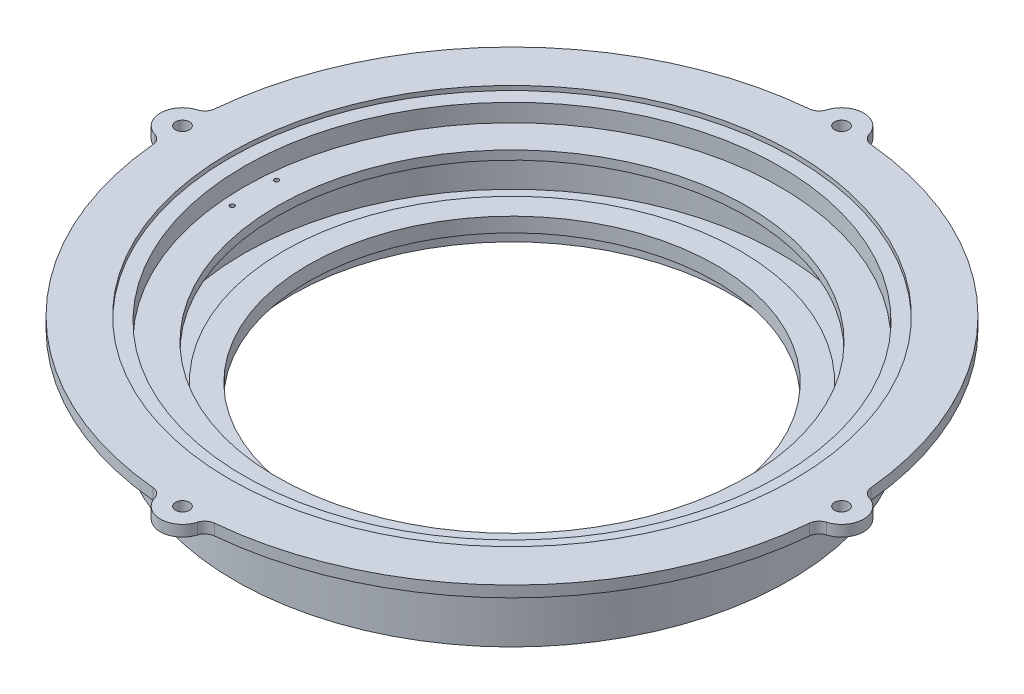
SolidWorks part; units mm, degrees
material "1060 合金"
ref_plane "Front Plane" through (0, 0, 0) normal (0, 0, 1) x (1, 0, 0)
ref_plane "Top Plane" through (0, 0, 0) normal (0, 1, 0) x (1, 0, 0)
ref_plane "Right Plane" through (0, 0, 0) normal (1, 0, 0) x (0, 0, -1)
sketch "Sketch1" plane through (0, 0, 0) normal (0, 0, 1) x (1, 0, 0)
  line L0 (0, 0) -> (0, -19.9402) construction
  line L1 (-125, 139.5) -> (-125, 175.5)
  line L2 (-125, 139.5) -> (-99, 139.5)
  line L3 (125, 139) -> (-125, 139) construction
  line L4 (-103, 144.5) -> (-103, 154.5)
  line L5 (-103, 154.5) -> (-92, 154.5)
  line L6 (-121, 180.5) -> (-148.7461, 180.5)
  line L7 (-148.7461, 180.5) -> (-148.7461, 175.5)
  line L8 (-148.7461, 175.5) -> (-125, 175.5)
  line L9 (-92, 154.5) -> (-92, 147.9626)
  line L10 (-92, 147.9626) -> (-99, 147.9626)
  line L11 (-99, 147.9626) -> (-99, 139.5)
  line L13 (-121, 170.5) -> (-106, 170.5)
  line L14 (-103, 144.5) -> (-121, 144.5)
  line L15 (-121, 144.5) -> (-121, 166.5)
  line L17 (-121, 166.5) -> (-106, 166.5)
  line L18 (-106, 170.5) -> (-106, 166.5)
  line L19 (-121, 170.5) -> (-121, 180.5)
  dimension "D1" = 15
  dimension "D2" = 4
  dimension "D3" = 12
  dimension "D4" = 10
  dimension "D5" = 0.5
revolve "Revolve1" add sketch "Sketch1" angle 360 about L0
sketch "Sketch2" plane through (0, 180.5, 0) normal (0, 1, 0) x (1, 0, 0)
  circle A0 centre (0, 0) radius 127.5
extrude "Cut-Extrude1" cut sketch "Sketch2" against normal blind 2
sketch "Sketch3" plane through (0, 175.5, 0) normal (0, -1, 0) x (1, 0, 0)
  circle A0 centre (0, -148.7461) radius 10
  circle A1 centre (0, 0) radius 148.7461 construction
  circle A2 centre (-148.7461, 0) radius 10
  circle A3 centre (0, 148.7461) radius 10
  circle A4 centre (148.7461, 0) radius 10
  point P13 (0, 0)
  dimension "D1" = 4
extrude "Boss-Extrude1" add sketch "Sketch3" against normal up to surface (5 mm away) up to face at (-127.5, 180.5, 0)
fillet "Fillet1" radius 5 8 edges at (9.9943, 178, 148.41) (-9.9943, 178, 148.41) (-148.41, 178, 9.9943) (-148.41, 178, -9.9943) (-9.9943, 178, -148.41) (9.9943, 178, -148.41) (148.41, 178, -9.9943) (148.41, 178, 9.9943)
sketch "Sketch4" plane through (0, 175.5, 0) normal (0, -1, 0) x (1, 0, 0)
  circle A0 centre (148.7461, 0) radius 3.15
  circle A1 centre (0, -148.7461) radius 3.15
  circle A2 centre (-148.7461, 0) radius 3.15
  circle A3 centre (0, 148.7461) radius 3.15
  point P12 (0, 0)
  dimension "D1" = 4
extrude "Cut-Extrude2" cut sketch "Sketch4" against normal blind 10
fillet "Fillet2" radius 7.5 1 edges at (-125, 175.5, 0)
sketch "Sketch5" plane through (0, 170.5, 0) normal (0, 1, 0) x (1, 0, 0)
  circle A0 centre (-116.2753, 10) radius 1
  circle A1 centre (-116.2753, -10) radius 1
  circle A2 centre (116.2753, 10) radius 1
  circle A3 centre (116.2753, -10) radius 1
extrude "Cut-Extrude3" cut sketch "Sketch5" against normal blind 5
